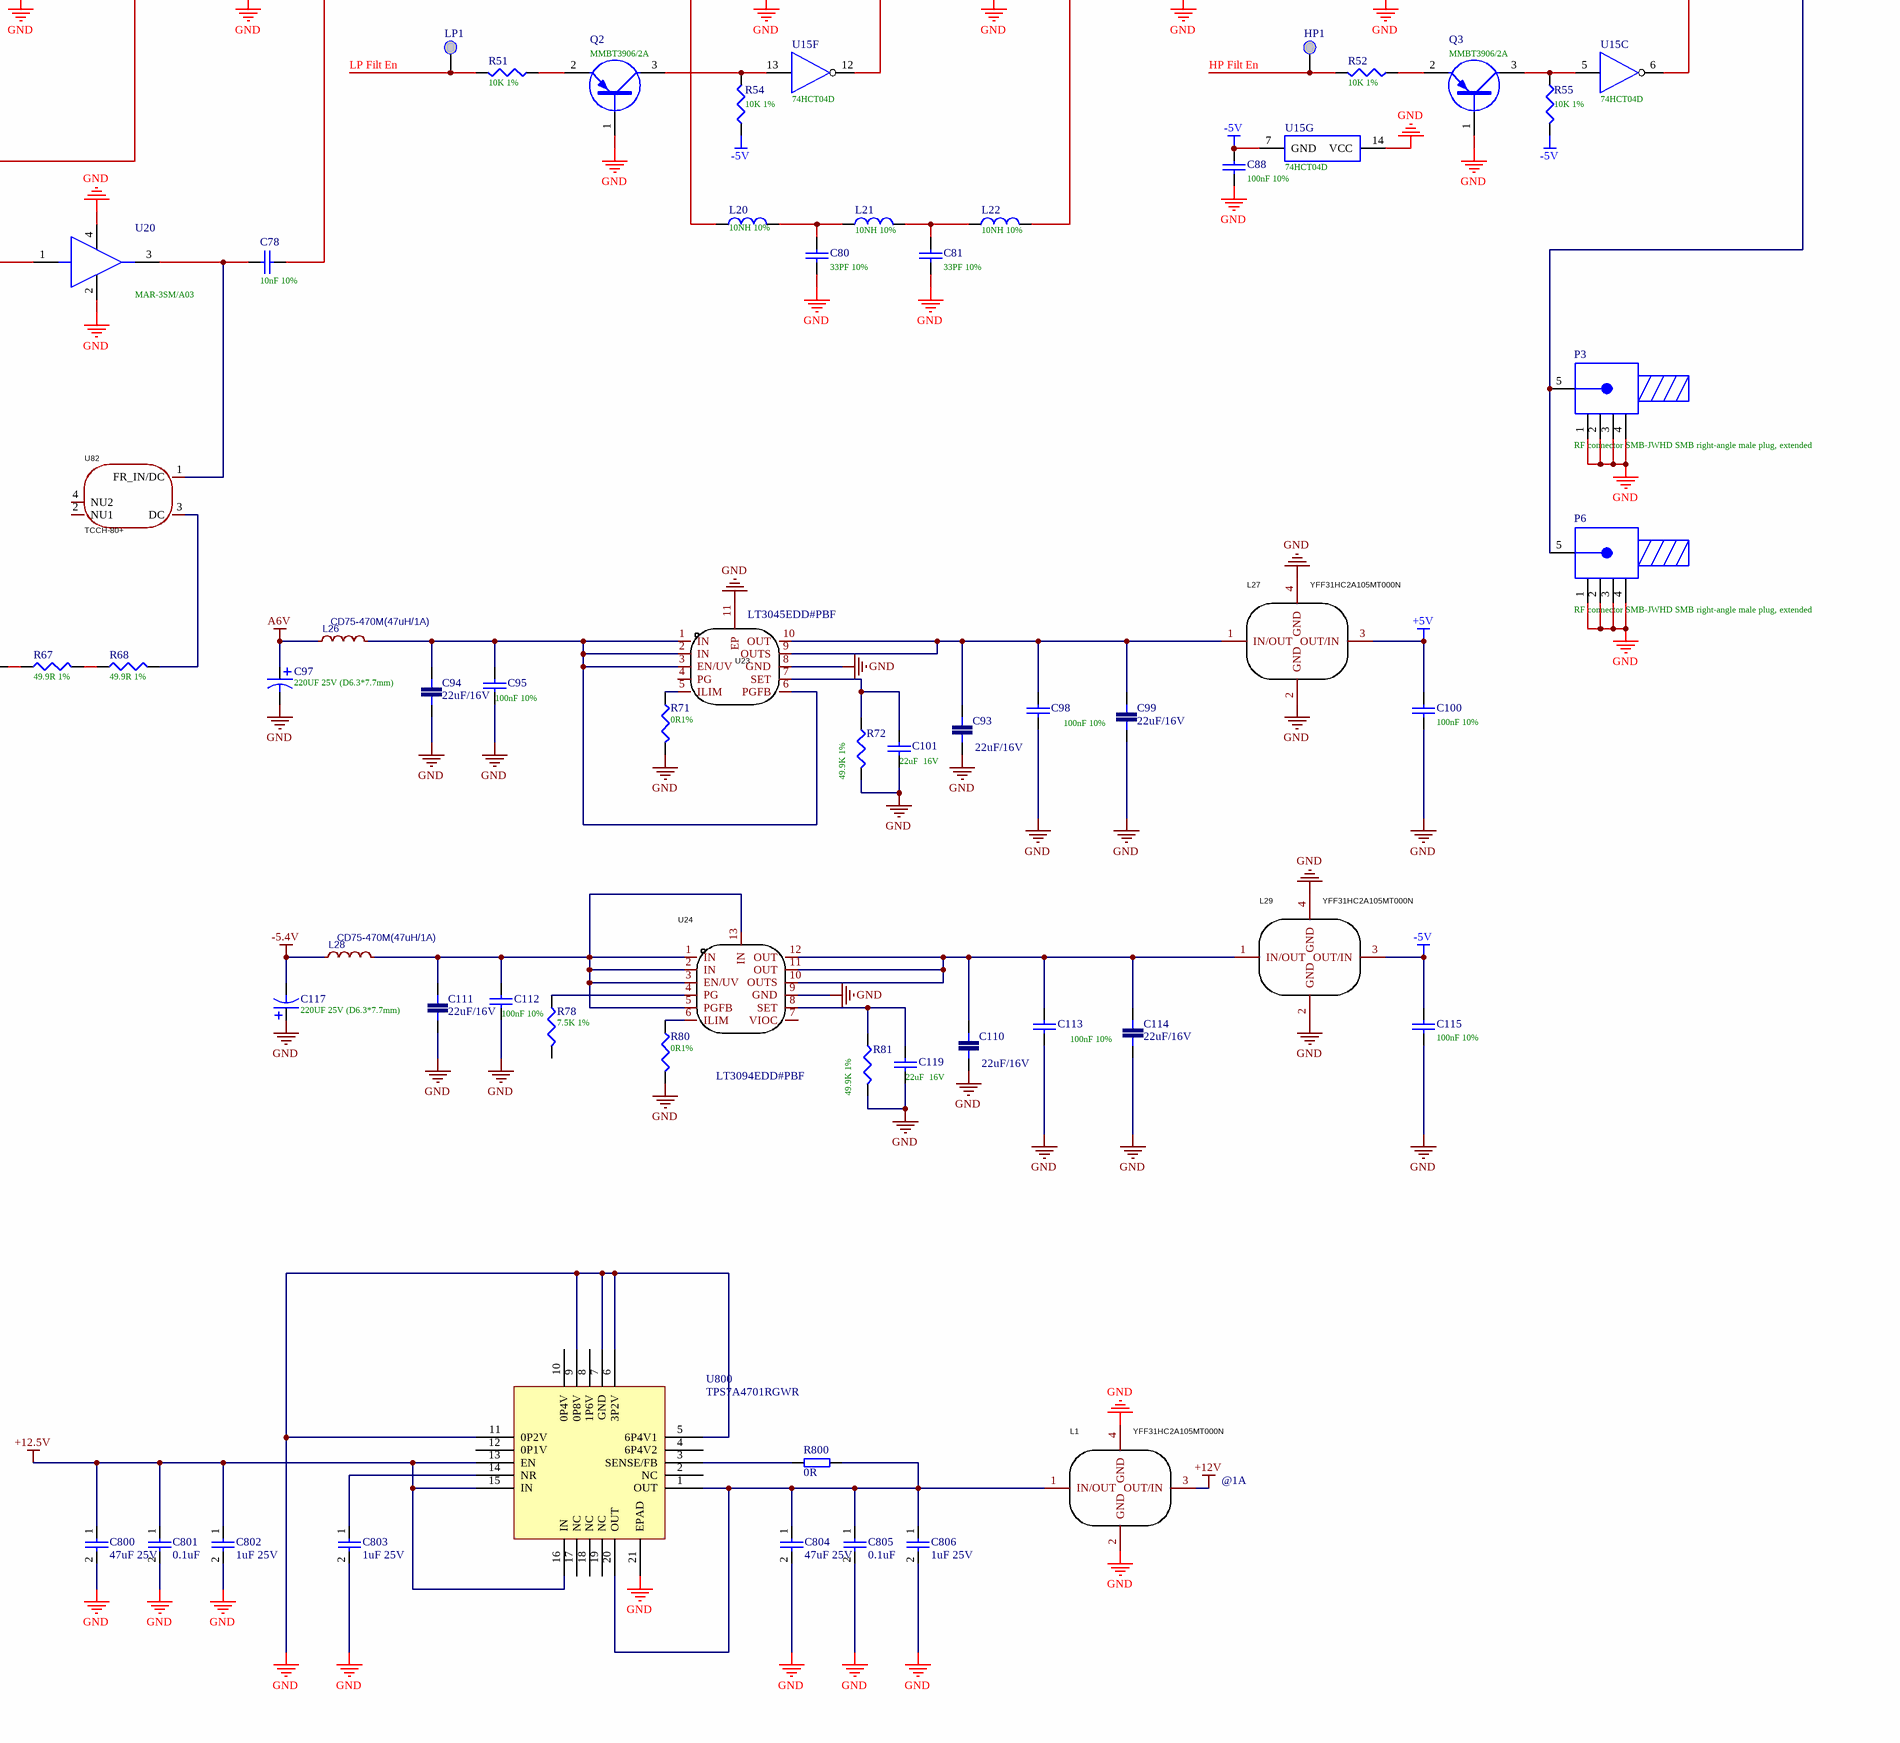
[diagram p0: PCBE109560-11.SchDoc, bottom right]
# Altium schematic sheet PCBE109560-11.SchDoc (part 2 of 2)

## Parts
1  (no value)  [DIP-1]
+1  (no value)  [DIP-1]
+2  (no value)  [DIP-1]
C4  20PF 10%  [0805C]
C5  330PF 10%  [1812C]
C6  22PF 10%  [1812C-2]
C7  22uF/16V  [0805]
C8  22uF/16V  [0805]
C9  100nF 10%  [0603]
C10  220UF 25V (D6.3*7.7mm)  [CAP-SMD_BD6.3-L6.6-W6.6-FD]
C11  100nF 10%  [0603]
C12  22uF/16V  [0805]
C13  100nF 10%  [0805R]
C14  22uF  16V  [0805]
C15  100nF 10%  [0805R]
C16  47PF 10%  [1812C-2]
C17  100PF 10%  [1812C-2]
C18  20PF 10%  [0805R]
C20  100nF 10%  [0805R]
C21  100nF 10%  [0805R]
C31  100nF 10%  [0805R]
C32  100nF 10%  [0805R]
C34  100nF 10%  [0805R]
C35  100nF 10%  [0805R]
C36  100nF 10%  [0805R]
C37  100nF 10%  [0805R]
C39  100nF 10%  [0805R]
C40  100nF 10%  [0805R]
C41  100nF 10%  [0805R]
C42  100nF 10%  [0805R]
C43  100nF 10%  [0805R]
C44  100nF 10%  [0805R]
C45  100nF 10%  [0805R]
C46  100nF 10%  [0805R]
C47  100nF 10%  [0805R]
C48  100nF 10%  [0805R]
C49  22uF 25V  [CAP-SMD_L6.0-W3.2-R-RD]
C50  100nF 10%  [0805R]
C51  100nF 10%  [0805R]
C52  100nF 10%  [0805R]
C53  3.3NF 10%  [0805R]
C54  100nF 10%  [0805R]
C55  330PF 10%  [0805R]
C56  330PF 10%  [0805R]
C57  100nF 10%  [0805R]
C58  33PF 10%  [0805R]
C59  33PF 10%  [0805R]
C60  100nF 10%  [0805R]
C61  100nF 10%  [0805R]
C62  100nF 10%  [0805R]
C63  100nF 10%  [0805R]
C64  100nF 10%  [0805R]
C65  33PF 10%  [0805R]
C66  33PF 10%  [0805R]
C67  100nF 10%  [0805R]
C68  39PF 10%  [0805R]
C69  100nF 10%  [0805R]
C70  25V 1UF Type A  [0805C-2]
C71  25V 1UF Type A  [0805C-2]
C72  100nF 10%  [0805R]
C73  25V 1UF Type A  [0805C-2]
C74  100nF 10%  [0805R]
C75  100nF 10%  [0805R]
C76  10nF 10%  [0805R]
C77  10nF 10%  [0805R]
C78  10nF 10%  [0805R]
C79  100nF 10%  [0603C]
C80  33PF 10%  [0805R]
C81  33PF 10%  [0805R]
C82  100nF 10%  [0805R]
C83  100nF 10%  [0805R]
C84  100nF 10%  [0805R]
C85  100nF 10%  [0805R]
C86  25V 1UF Type A  [0805C-2]
C87  3pF( ±0.1pF)  [0805R]
C88  100nF 10%  [0805R]
C89  100nF 10%  [0805R]
C90  100nF 10%  [0805R]
C93  22uF/16V  [0805]
C94  22uF/16V  [0805]
C95  100nF 10%  [0603]
C96  100nF 10%  [0805R]
C97  220UF 25V (D6.3*7.7mm)  [CAP-SMD_BD6.3-L6.6-W6.6-FD]
C98  100nF 10%  [0603]
C99  22uF/16V  [0805]
C100  100nF 10%  [0805R]
C101  22uF  16V  [0805]
C102  100nF 10%  [0805R]
C103  100nF 10%  [0805R]
C104  100nF 10%  [0805R]
C105  100nF 10%  [0805R]
C106  100nF 10%  [0805R]
C107  100nF 10%  [0805R]
C109  100nF 10%  [0805R]
C110  22uF/16V  [0805]
C111  22uF/16V  [0805]
C112  100nF 10%  [0603]
C113  100nF 10%  [0603]
C114  22uF/16V  [0805]
C115  100nF 10%  [0805R]
C116  100nF 10%  [0805R]
C117  220UF 25V (D6.3*7.7mm)  [CAP-SMD_BD6.3-L6.6-W6.6-FD]
C118  100nF 10%  [0805R]
C119  22uF  16V  [0805]
C122  100nF 10%  [0805R]
C123  100nF 10%  [0805R]
C124  100nF 10%  [0805R]
C125  100nF 10%  [0805R]
C128  100nF 10%  [0805R]
C129  100nF 10%  [0805R]
C130  100nF 10%  [0805R]
C800  47uF 25V  [1206]
C801  0.1uF  [0402]
C802  1uF 25V  [0402]
C803  1uF 25V  [0402]
C804  47uF 25V  [1206]
C805  0.1uF  [0402]
C806  1uF 25V  [0402]
C809  100nF 10%  [0805R]
C888  100nF 10%  [0805R]
Clk1  (no value)  [DIP-1]
D1  BAV99/A7  [SOT-23]
D2  GF1M-E3/67A/GM  [1808D]
D3  GF1M-E3/67A/GM  [1808D]
D4  GF1M-E3/67A/GM  [1808D]
D5  GF1M-E3/67A/GM  [1808D]
D8  BAV99/A7  [SOT-23-2]
D9  BAV99/A7  [SOT-23-2]
D10  BAV99/A7  [SOT-23-2]
D11  BAV99/A7  [SOT-23-2]
D12  BAV99/A7  [SOT-23-2]
Data1  (no value)  [DIP-1]
HP1  (no value)  [DIP-1]
J1  RF connector  [DIP-P]
J2  RF connector  [DIP-P]
L1  YFF31HC2A105MT000N  [FILTER-SMD_4P-L3.2-W1.6-L_YFF31HC]
L2  15UH 5%  [1005R]
L3  BLM21PG221SN1D(220Ω@100MHz)  [0805R]
L4  YFF31HC2A105MT000N  [FILTER-SMD_4P-L3.2-W1.6-L_YFF31HC]
L5  6.8UH 10%  [0805R]
L8  YFF31HC2A105MT000N  [FILTER-SMD_4P-L3.2-W1.6-L_YFF31HC]
L10  10NH 10%  [0805R]
L11  10NH 10%  [0805R]
L12  10NH 10%  [0805R]
L13  YFF31HC2A105MT000N  [FILTER-SMD_4P-L3.2-W1.6-L_YFF31HC]
L15  4.7UH 5%  [1005L]
L16  1UH 5%  [0805R]
L17  BLM21PG221SN1D(220Ω@100MHz)  [0805R]
L18  BLM21PG221SN1D(220Ω@100MHz  [0805R]
L19  NFM15PC104R1A3D  [FILTER-SMD_0402-3P-L1.0-W0.5-T]
L20  10NH 10%  [0805R]
L21  10NH 10%  [0805R]
L22  10NH 10%  [0805R]
L23  YFF31HC2A105MT000N  [FILTER-SMD_4P-L3.2-W1.6-L_YFF31HC]
L24  YFF31HC2A105MT000N  [FILTER-SMD_4P-L3.2-W1.6-L_YFF31HC]
L25  BLM21PG221SN1D(220Ω@100MHz  [0805R]
L26  CD75-470M(47uH/1A)  [IND-SMD_L7.8-W7.0-A]
L27  YFF31HC2A105MT000N  [FILTER-SMD_4P-L3.2-W1.6-L_YFF31HC]
L28  CD75-470M(47uH/1A)  [IND-SMD_L7.8-W7.0-A]
L29  YFF31HC2A105MT000N  [FILTER-SMD_4P-L3.2-W1.6-L_YFF31HC]
L31  BLM21PG221SN1D(220Ω@100MHz  [0805R]
L32  BLM21PG221SN1D(220Ω@100MHz  [0805R]
L808  NFM15PC104R1A3D  [FILTER-SMD_0402-3P-L1.0-W0.5-T]
L809  NFM15PC104R1A3D  [FILTER-SMD_0402-3P-L1.0-W0.5-T]
L810  NFM15PC104R1A3D  [FILTER-SMD_0402-3P-L1.0-W0.5-T]
L811  NFM15PC104R1A3D  [FILTER-SMD_0402-3P-L1.0-W0.5-T]
L812  NFM15PC104R1A3D  [FILTER-SMD_0402-3P-L1.0-W0.5-T]
L813  NFM15PC104R1A3D  [FILTER-SMD_0402-3P-L1.0-W0.5-T]
LP1  (no value)  [DIP-1]
P1  Header 20X2  [N0.8mm/40Pin-Plug]
P2  Header 4X2  [N0.8mm/8Pin-SOCKET]
P3  RF connector SMB-JWHD SMB right-angle male plug, extended  [DIP-P-2]
P4  Header 20X2  [N0.8mm/40Pin-Plug]
P5  Header 20X2  [N0.8mm/40Pin-Plug]
P6  RF connector SMB-JWHD SMB right-angle male plug, extended  [DIP-P-2]
Q1  MJD31C  [SOT-252-2]
Q2  MMBT3906/2A  [SOT-23]
Q3  MMBT3906/2A  [SOT-23]
Q4  MMBT3906/2A  [SOT-23]
R6  2K 5%  [0603R]
R7  NC  [AXIAL-0.51]
R8  3.9K 5% 1/2W  [AXIAL-0.51]
R9  3.9K 5% 1/2W  [AXIAL-0.51]
R10  3.9K 5% 1/2W  [AXIAL-0.51]
R11  3.9K 5% 1/2W  [AXIAL-0.51]
R13  0R1%  [0603]
R14  49.9K 1%  [0603]
R15  4.99K 1%  [0805R]
R16  2K 1%  [0805R]
R17  49.9R 1% 1/4W  [AXIAL-0.4]
R20  100R 1% 1/4W  [AXIAL-0.4]
R23  100R 1% 1/4W  [AXIAL-0.4]
R27  4.87K 1%  [0805R]
R28  4.87K 1%  [0805R]
R29  4.87K 1%  [0805R]
R30  4.87K 1%  [0805R]
R31  4.87K 1%  [0805R]
R32  10K 1%  [0805R]
R33  100K 1%  [0805R]
R34  100K 1%  [0805R]
R35  49.9R 1%  [0805R]
R36  49.9R 1%  [0805R]
R37  49.9R 1%  [0805R]
R38  49.9R 1%  [0805R]
R39  49.9R 1%  [0805R]
R40  49.9R 1% 1/4W  [R-SMD_L3.5-W1.5]
R41  10K 1%  [0805R]
R42  4.87K 1%  [0805R]
R43  4.87K 1%  [0805R]
R44  4.87K 1%  [0805R]
R45  4.87K 1%  [0805R]
R46  169R 1%  [0805R]
R47  169R 1%  [0805R]
R48  169R 1%  [0805R]
R49  49.9R 1%  [0805R]
R50  49.9R 1%  [0805R]
R51  10K 1%  [0805R]
R52  10K 1%  [0805R]
R53  10K 1%  [0805R]
R54  10K 1%  [0805R]
R55  10K 1%  [0805R]
R56  10K 1%  [0805R]
R57  10K 1%  [0805R]
R58  49.9R 1%  [0805R]
R59  4.99K 1%  [0805R]
R60  49.9R 1%  [R-SMD_L3.5-W1.5]
R61  30R 1%  [R-SMD_L3.5-W1.5]
R62  169R 1%  [0805R]
R63  169R 1%  [0805R]
R64  169R 1%  [0805R]
R65  49.9R 1%  [0805R]
R66  49.9R 1%  [0805R]
R67  49.9R 1%  [0805R]
R68  49.9R 1%  [0805R]
R69  120R 1%  [R-SMD_L3.5-W1.5]
R70  169R 1%  [0805R]
R71  0R1%  [0603]
R72  49.9K 1%  [0603]
R73  169R 1%  [0805R]
R74  NC  [0805R]
R75  169R 1%  [0805R]
R77  169R 1%  [0805R]
R78  7.5K 1%  [0603]
R80  0R1%  [0603]
R81  49.9K 1%  [0603]
R82  100K 1%  [0805R]
R83  10K 1%  [0805R]
R84  169R 1%  [0805R]
R800  0R  [0402]
RE1  AGQ210A4HZ  [RELAY-SMD_PANASONIC_AGQ2X0AXX]
RE2  AGQ210A4HZ  [RELAY-SMD_PANASONIC_AGQ2X0AXX]
RE3  AGQ210A4HZ  [RELAY-SMD_PANASONIC_AGQ2X0AXX]
RE4  AGQ210A4HZ  [RELAY-SMD_PANASONIC_AGQ2X0AXX]
RE5  AGQ210A4HZ  [RELAY-SMD_PANASONIC_AGQ2X0AXX]
Strobe1  (no value)  [DIP-1]
U4  LT3045EDD#PBF  [DFN-10_L3.0-W3.0-P0.50-BL-EP]
U6  74HCT123D  [SOIC-16_L9.9-W3.9-P1.27-LS6.0-BL]
U8  MAX504CSD+T  [SO-14]
U9  SW-239  [SO-8]
U11  SW-239  [SO-8]
U12  SW-239  [SO-8]
U13  SW-239  [SO-8]
U14  SW-239  [SO-8]
U15  74HCT04D  [SO-14]  (parts A,B,C,D,E,F,G of 7)
U16  AT-250(MAAV-007941)  [SO-8]
U17  MAR-3SM/A03  [LCC4]
U18  MAR-6SM/A06  [LCC4]
U19  MAR-6SM/A06  [LCC4]
U20  MAR-3SM/A03  [LCC4]
U21  MAX4106ESA+T  [SO-8]
U22  MIC4420CM  [SO-8]
U23  LT3045EDD#PBF  [DFN-10_L3.0-W3.0-P0.50-BL-EP]
U24  LT3094EDD#PBF  [WDFN-12_L3.0-W3.0-P0.45-BL-EP]
U25  AT65-0263  [SO-16]
U80  TCCH-80+  [IND-SMD_4P-L3.8-W3.8]
U81  TCCH-80+  [IND-SMD_4P-L3.8-W3.8]
U82  TCCH-80+  [IND-SMD_4P-L3.8-W3.8]
U83  TCCH-80+  [IND-SMD_4P-L3.8-W3.8]
U100  SW-239  [SO-8]
U800  TPS7A4701RGWR  [QFN-20]

## Nets
+5V: C100.1 C888.1 L25.1 L27.3(OUT/IN) L811.3(OUTPUT) L812.3(OUTPUT) U8.3(~{CLR})
+12.5V: +2.1 C106.1 C800.1 C801.1 C802.1 P5.31 P5.32 P5.33 P5.34 P5.35 P5.36 P5.37 P5.38 P5.39 P5.40 U800.13(EN) U800.15(IN) U800.16(IN)
+12V: C122.1 C123.1 C124.2 C125.2 L1.3(OUT/IN) L8.1(IN/OUT) L13.1(IN/OUT) U22.1(VS) U22.8(VS)
-5.4V: +1.1 C107.1 C117.2 L28.2 P5.1 P5.2 P5.3 P5.4 P5.5 P5.6 P5.7 P5.8 P5.9 P5.10
-5V: C88.2 C115.2 L29.3(OUT/IN) L809.1(INPUT) L810.3(OUTPUT) L813.3(OUTPUT) R54.1 R55.2 R57.1 U15.7(GND)
A6V: 1.1 C10.1 C97.1 C103.2 L3.1 L26.2 P5.17 P5.18 P5.19 P5.20 P5.21 P5.22 P5.23 P5.24
GND: C5.1 C6.2 C7.1 C8.1 C9.2 C10.2 C11.2 C12.1 C13.2 C14.2 C15.1 C18.2 C20.1 C21.1 C31.1 C32.1 C34.1 C35.1 C36.2 C37.2 C39.2 C40.2 C42.2 C43.1 C44.2 C45.2 C46.2 C47.1 C48.1 C49.2 C50.2 C57.2 C60.2 C61.1 C62.1 C63.1 C64.1 C65.2 C66.1 C70.1 C71.1 C72.2 C73.1 C74.1 C75.1 C80.1 C81.1 C83.2 C84.2 C85.1 C86.2 C88.1 C89.2 C90.2 C93.1 C94.1 C95.2 C96.2 C97.2 C98.2 C99.1 C100.2 C101.2 C102.2 C103.1 C104.2 C105.1 C106.2 C107.2 C109.2 C110.1 C111.1 C112.2 C113.2 C114.1 C115.1 C117.1 C118.2 C119.2 C122.2 C123.2 C124.1 C125.1 C128.1 C129.1 C130.2 C800.2 C801.2 C802.2 C803.2 C804.2 C805.2 C806.2 C809.2 C888.2 D1.3 D2.2(K) D11.2 D12.1 J1.1 J1.2 J1.3 J1.4 J2.1 J2.2 J2.3 J2.4 L1.2(GND) L1.4(GND) L2.2 L4.2(GND) L4.4(GND) L8.2(GND) L8.4(GND) L13.2(GND) L13.4(GND) L15.2 L16.1 L19.2(GND) L23.2(GND) L23.4(GND) L24.2(GND) L24.4(GND) L27.2(GND) L27.4(GND) L29.2(GND) L29.4(GND) L808.2(GND) L809.2(GND) L810.2(GND) L811.2(GND) L812.2(GND) L813.2(GND) P1.5 P1.6 P1.11 P1.12 P1.17 P1.18 P1.20 P1.23 P1.24 P1.29 P1.30 P1.35 P1.36 P2.1 P2.3 P2.5 P2.7 P3.1 P3.2 P3.3 P3.4 P4.5 P4.6 P4.11 P4.12 P4.17 P4.18 P4.23 P4.24 P4.29 P4.30 P4.35 P4.36 P5.11 P5.12 P5.13 P5.14 P5.15 P5.16 P5.25 P5.26 P5.27 P5.28 P5.29 P5.30 P6.1 P6.2 P6.3 P6.4 Q1.2(E) Q2.1(B) Q3.1(B) Q4.1(B) R13.2 R14.2 R20.2 R32.2 R53.1 R59.1 R61.1 R71.2 R72.2 R74.1 R80.2 R81.2 R82.1 R83.1 RE1.3 RE3.6 RE4.2 U4.8(GND) U4.11(EP) U6.6(2CEXT) U6.8(GND) U6.10(2B) U6.14(1CEXT) U8.7(DGND) U8.8(AGND) U9.2(GND) U9.7(GND) U9.8(GND) U11.2(GND) U11.7(GND) U11.8(GND) U12.2(GND) U12.7(GND) U12.8(GND) U13.2(GND) U13.7(GND) U13.8(GND) U14.2(GND) U14.7(GND) U14.8(GND) U15.14(VCC) U16.2(GND) U16.3(GND) U16.5(GND) U16.6(GND) U16.7(GND) U17.2(GND) U17.4(GND) U18.2(GND) U18.4(GND) U19.2(GND) U19.4(GND) U20.2(GND) U20.4(GND) U22.4(GND) U22.5(GND) U23.8(GND) U23.11(EP) U24.9(GND) U25.2(GND) U25.3(GND) U25.4(GND) U25.5(GND) U25.6(GND) U25.7(GND) U25.16(GND) U100.2(GND) U100.7(GND) U100.8(GND) U800.5(6P4V1) U800.6(3P2V) U800.7(GND) U800.9(0P8V) U800.11(0P2V) U800.21(EPAD)
VCC: C13.1 C15.2 L4.3(OUT/IN) R15.1 R16.2 U6.2(1B) U6.3(1~{R}D) U6.16(VCC)
AK2: C21.2 P1.33 RE1.1
AK3: C20.2 P1.38 RE1.8
AK4: C37.1 P1.37 RE2.1
AK5: C36.1 P1.40 RE2.8
AK6: C31.2 P1.34 RE3.8
AK7: C32.2 P1.32 RE3.1
AK8: C34.2 C40.1 P1.28 RE4.8 RE5.8
AK9: C35.2 C39.1 P1.26 RE4.1 RE5.1
Attn1: P4.34 R70.2
Attn2: P4.32 R73.2
Attn4: P4.28 R75.2
Attn8: P4.26 R77.2
Attn16: P4.22 R84.2
DAC Clk: Clk1.1 P4.14 U8.4(SCLK)
DAC Data: Data1.1 P4.16 U8.2(DIN)
DAC Strobe: P4.10 Strobe1.1 U8.5(~{CS})
DATA_T: P1.39 R15.2 U6.1(1~{A})
HP Filt En: HP1.1 P4.4 R52.2
HT: L5.1 P2.2 P2.4 P2.6 P2.8
IN2: P4.8 R56.1 U22.2(IN)
LP Filt En: LP1.1 P4.2 R51.2
NetC4_1: C4.1 D1.2 L2.1 Q1.1(B) R6.1
NetC4_2: C4.2 R6.2 U6.13(1Q)
NetC5_2: C5.2 L5.2 R7.2
NetC6_1: C6.1 C16.2 C17.2 Q1.3(C) R11.1
NetC7_2: C7.2 C11.1 C12.2 L4.1(IN/OUT) U4.9(OUTS) U4.10(OUT)
NetC8_2: C8.2 C9.1 L3.2 U4.1(IN) U4.2(IN) U4.3(EN/UV) U4.6(PGFB)
NetC14_1: C14.1 R14.1 U4.7(SET)
NetC16_1: C16.1 D5.1(A) D8.2 D9.2 RE2.6
NetC17_1: C17.1 RE2.7
NetC18_1: C18.1 R16.1 U6.15(1REXT/CEXT)
NetC41_1: C41.1 U14.1(RFCOM)
NetC41_2: C41.2 P3.5 P6.5 R32.1
NetC42_1: C42.1 R27.1 U9.5(B)
NetC43_2: C43.2 R28.2 U100.4(A)
NetC44_1: C44.1 R29.1 U11.4(A)
NetC45_1: C45.1 R30.1 U12.5(B)
NetC46_1: C46.1 R31.1 U13.5(B) U14.4(A)
NetC47_2: C47.2 R35.1 U16.4(A)
NetC48_2: C48.2 L8.3(OUT/IN) R36.1
NetC49_1: C49.1 C50.1 U8.1(BIPOFF) U8.9(REFIN) U8.10(REFOUT)
NetC51_1: C51.1 U17.1(RF_IN)
NetC51_2: C51.2 U16.8(RF2)
NetC52_1: C52.1 L10.2
NetC52_2: C52.2 U17.3(RF_OUT) U81.1(FR_IN/DC)
NetC53_1: C53.1 C54.1 L15.1
NetC53_2: C53.2 U12.1(RFCOM)
NetC54_2: C54.2 U13.1(RFCOM)
NetC55_1: C55.1 U13.3(RF1)
NetC55_2: C55.2 C56.1 L16.2
NetC56_2: C56.2 U14.6(RF2)
NetC57_1: C57.1 R41.1 U13.4(A) U14.5(B)
NetC58_1: C58.1 C65.1
NetC58_2: C58.2 L10.1 L11.1
NetC59_1: C59.1 L11.2 L12.1
NetC59_2: C59.2 C66.2
NetC60_1: C60.1 R42.1 U9.4(A)
NetC61_2: C61.2 R43.2 U100.5(B)
NetC62_2: C62.2 R44.1 U11.5(B)
NetC63_2: C63.2 R45.1 U12.4(A)
NetC64_2: C64.2 L13.3(OUT/IN) R46.2
NetC67_1: C67.1 U18.1(RF_IN)
NetC67_2: C67.2 U25.1(RF)
NetC68_1: C68.1 C69.2 R49.2 R50.2
NetC68_2: C68.2 R49.1 R50.1 U18.3(RF_OUT) U80.1(FR_IN/DC)
NetC69_1: C69.1 R53.2 U16.1(RF1)
NetC70_2: C70.2 C74.2 L18.1 L19.1(INPUT)
NetC71_2: C71.2 C75.2 L19.3(OUTPUT) U21.4(VEE)
NetC72_1: C72.1 C73.2 L17.2 L18.2
NetC76_1: C76.1 U9.3(RF1)
NetC76_2: C76.2 U19.1(RF_IN)
NetC77_1: C77.1 U19.3(RF_OUT) U83.1(FR_IN/DC)
NetC77_2: C77.2 U20.1(RF_IN)
NetC78_1: C78.1 U20.3(RF_OUT) U82.1(FR_IN/DC)
NetC78_2: C78.2 U100.6(RF2)
NetC79_1: C79.1 D10.3 R40.2
NetC79_2: C79.2 R58.2 R59.2
NetC80_2: C80.2 L20.2 L21.2
NetC81_2: C81.2 L21.1 L22.1
NetC82_1: C82.1 R60.2
NetC82_2: C82.2 C116.1 R74.2 R82.2
NetC83_1: C83.1 C86.1 L808.1(INPUT) U21.7(VCC)
NetC84_1: C84.1 L23.3(OUT/IN) R62.2
NetC85_2: C85.2 L24.3(OUT/IN) R65.1
NetC87_1: C87.1 R60.1 R69.1 U21.6(OUT)
NetC87_2: C87.2 R61.2 R69.2 U21.2(IN-)
NetC89_1: C89.1 L813.1(INPUT) U8.11(VSS)
NetC90_1: C90.1 L32.2 L811.1(INPUT)
NetC93_2: C93.2 C98.1 C99.2 L27.1(IN/OUT) U23.9(OUTS) U23.10(OUT)
NetC94_2: C94.2 C95.1 L26.1 U23.1(IN) U23.2(IN) U23.3(EN/UV) U23.6(PGFB)
NetC96_1: C96.1 R70.1 U25.15(C1)
NetC101_1: C101.1 R72.1 U23.7(SET)
NetC102_1: C102.1 R73.1 U25.14(C2)
NetC104_1: C104.1 L812.1(INPUT) U8.13(VDD)
NetC105_2: C105.2 L31.1 L810.1(INPUT)
NetC109_1: C109.1 R75.1 U25.13(C4)
NetC110_2: C110.2 C113.1 C114.2 L29.1(IN/OUT) U24.10(OUTS) U24.11(OUT) U24.12(OUT)
NetC111_2: C111.2 C112.1 L28.1 U24.1(IN) U24.2(IN) U24.3(EN/UV) U24.5(PGFB) U24.13(IN)
NetC116_2: C116.2 R83.2 U25.8(RF)
NetC118_1: C118.1 R77.1 U25.12(C8)
NetC119_1: C119.1 R81.1 U24.8(SET)
NetC128_2: C128.2 L31.2 U25.11(VEE)
NetC129_2: C129.2 L32.1 U25.10(VCC)
NetC130_1: C130.1 R84.1 U25.9(C16)
NetC803_1: C803.1 U800.14(NR)
NetC804_1: C804.1 C805.1 C806.1 L1.1(IN/OUT) R800.1 U800.1(OUT) U800.20(OUT)
NetC809_1: C809.1 L25.2 L808.3(OUTPUT)
NetD2_1: D2.1(A) D3.2(K)
NetD3_1: D3.1(A) D4.2(K)
NetD4_1: D4.1(A) D5.2(K)
NetD8_1: D8.1 D9.1 J1.5 R17.1 R20.1 R23.1 RE4.4
NetD10_1: D10.1 D12.2
NetD10_2: D10.2 D11.1
NetJ2_5: J2.5 RE5.4
NetL12_2: L12.2 U9.1(RFCOM)
NetL17_1: L17.1 L809.3(OUTPUT)
NetL20_1: L20.1 U11.6(RF2)
NetL22_2: L22.2 U12.3(RF1)
NetL23_1: L23.1(IN/OUT) L24.1(IN/OUT) U22.6(OUT) U22.7(OUT)
NetQ2_2: Q2.2(E) R51.1
NetQ2_3: Q2.3(C) R54.2 U15.13(6A)
NetQ3_2: Q3.2(E) R52.1
NetQ3_3: Q3.3(C) R55.1 U15.5(3A)
NetQ4_2: Q4.2(E) R56.2
NetQ4_3: Q4.3(C) R57.2 U15.1(1A)
NetR7_1: R7.1 R8.1
NetR8_2: R8.2 R9.2
NetR9_1: R9.1 R10.1
NetR10_2: R10.2 R11.2
NetR13_1: R13.1 U4.5(ILIM)
NetR17_2: R17.2 RE1.2
NetR23_2: R23.2 RE3.7
NetR27_2: R27.2 R28.1 U15.4(2Y)
NetR29_2: R29.2 R30.2 U15.10(5Y)
NetR31_2: R31.2 U15.8(4Y)
NetR33_1: R33.1 R34.1 U8.14(RFB)
NetR33_2: R33.2 R34.2 R35.2 U8.12(VOUT)
NetR36_2: R36.2 R37.1
NetR37_2: R37.2 R38.2
NetR38_1: R38.1 R39.1
NetR39_2: R39.2 U81.3(DC)
NetR40_1: R40.1 RE5.3
NetR41_2: R41.2 U15.6(3Y) U15.9(4A)
NetR42_2: R42.2 R43.1 U15.2(1Y) U15.3(2A)
NetR44_2: R44.2 R45.2 U15.11(5A) U15.12(6Y)
NetR46_1: R46.1 R47.2
NetR47_1: R47.1 R48.1
NetR48_2: R48.2 U80.3(DC)
NetR58_1: R58.1 U21.3(IN+)
NetR62_1: R62.1 R63.1
NetR63_2: R63.2 R64.2
NetR64_1: R64.1 U83.3(DC)
NetR65_2: R65.2 R66.2
NetR66_1: R66.1 R67.1
NetR67_2: R67.2 R68.1
NetR68_2: R68.2 U82.3(DC)
NetR71_1: R71.1 U23.5(ILIM)
NetR78_1: R78.1 U24.4(PG)
NetR80_1: R80.1 U24.6(ILIM)
NetR800_2: R800.2 U800.3(SENSE/FB)
NetRE4_3: RE4.3 RE5.2
NetU9_6: U9.6(RF2) U100.3(RF1)
NetU11_1: U11.1(RFCOM) U100.1(RFCOM)
NetU11_3: U11.3(RF1) U12.6(RF2)
NetU13_6: U13.6(RF2) U14.3(RF1)

Not connected (* = marked no-connect by the designer): D1 1*; D8 3; D9 3; D11 3; D12 3; P1 1 2 3 4 7 8 9 10 13 14 15 16 19 21 22 25 27 31; P4 1 3 7 9 13 15 19 20 21 25 27 31 33 37 38 39 40; R78 2; RE1 4 5 6 7; RE2 2 3 4 5; RE3 2 3 4 5; RE4 5 6 7; RE5 5 6 7; U4 4(PG); U6 4(1~{Q}) 5(2Q) 7(2REXT/CEXT) 9(2~{A}) 11(2~{R}D) 12(2~{Q}); U8 6(DOUT); U22 3(NC); U23 4(PG); U24 7(VIOC); U80 2(NU1) 4(NU2); U81 2(NU1) 4(NU2); U82 2(NU1) 4(NU2); U83 2(NU1) 4(NU2); U800 2(NC) 4(6P4V2) 8(1P6V) 10(0P4V) 12(0P1V) 17(NC) 18(NC) 19(NC)

## Notes on the sheet
- (near P1) Transmit interface
- 500V high-voltage interface
- Receive interface
- @1A

## Library data of the parts
1 +1 +2 Clk1 Data1 HP1 LP1 Strobe1 = TP
C4-C6 C9 C11 C13-C18 C20 C21 C31 C32 C34-C37 C39-C48 C50-C69 C72-C85 C87-C90 C95 C96 C98 C100-C107 C109 C112 C113 C115 C116 C118 C119 C122-C125 C128-C130 C800-C806 C809 C888 = CAP: Capacitor
C7 C8 C12 C93 C94 C99 C110 C111 C114 = C1206
C10 C97 C117 = CAPACITOR_1: Capacitor
C49 = TAJC226K025RNJ: Manufacturer: Kyocera AVX; Add into BOM: yes; Tolerance: ±10%; Equivalent Series Resistance(ESR): 1.4Ω@100kHz; Symbol: TAJC226K025RNJ; Device: TAJC226K025RNJ; LCSC Part Name: 22uF ±10% 25V; Supplier Part: C7214; Manufacturer Part: TAJC226K025RNJ; Supplier Footprint: CASE-C-6032; JLCPCB Part Class: Extended Part; Datasheet: https://atta.szlcsc.com/upload/public/pdf/source/20160107/1457707750344.pdf; Supplier: LCSC; Convert to PCB: yes; Value: 22uF; Rated Voltage: 25V; Operating Temperature: -55℃~+125℃
C70 C71 C86 = CAPACITOR POL: Capacitor
D1 D8-D12 = BAV99
D2-D5 = DIODE
J1 J2 = SMA-KWE: BOM_Supplier: *; BOM_Supplier Part: *; BOM_Manufacturer: *; BOM_Manufacturer Part: *; BOM_JLCPCB Part Class: *; spicePre: *; spiceSymbolName: *; Contributor: *
L1 L4 L8 L13 L23 L24 L27 L29 = YFF31HC2A105MT000N: Manufacturer: TDK; Add into BOM: yes; Nominal Capacitance: 1uF; CapacitanceTolerance: ±20%; DC Rated Voltage: 100V; Rated Current: 6A; DC Resistance: 5mΩ; Name: YFF31HC2A105MT000N; Symbol: YFF31HC2A105MT000N; Device: YFF31HC2A105MT000N; LCSC Part Name: 1uF(105) ±20% 100V; Supplier Part: C113216; Manufacturer Part: YFF31HC2A105MT000N; Supplier Footprint: SMD-4P,1.6x3.2mm; JLCPCB Part Class: Extended Part; Datasheet: https://atta.szlcsc.com/upload/public/pdf/source/20180326/C113216_F6F81E50B9805DA3D7C436129903DEBD.pdf; Supplier: LCSC; Convert to PCB: yes; Operating Temperature: -55℃~+125℃
L2 L3 L5 L10-L12 L15-L18 L20-L22 L25 L31 L32 = INDUCTOR
L19 L808-L813 = NFM15PC104R1A3D: Manufacturer: muRata(村田); Add into BOM: yes; Nominal Capacitance: 100nF; CapacitanceTolerance: ±20%; DC Rated Voltage: 10V; Rated Current: 2A; DC Resistance: 30mΩ; Symbol: NFM15PC104R1A3D; Device: NFM15PC104R1A3D; LCSC Part Name: 0.1uF ±20% 10V; Supplier Part: C2650905; Manufacturer Part: NFM15PC104R1A3D; Supplier Footprint: 0402; JLCPCB Part Class: Extended Part; Datasheet: https://atta.szlcsc.com/upload/public/pdf/source/20210611/05FD8D968916F804F398094FB2B4AAFE.pdf; Supplier: LCSC; Convert to PCB: yes; Operating Temperature: -55℃~+105℃; Comment_1: NFM15PC104R1A3D
L26 L28 = 4.7uH/5a: BOM_Manufacturer: COILMX; BOM_Manufacturer Part: MS0630-4R7M; nameAlias: Inductance; Contributor: LCSC; BOM_Supplier: LCSC; BOM_Supplier Part: C380177; spicePre: L; spiceSymbolName: MS0630-4R7M
P1 P4 P5 = Header 20X2: Header, 20-Pin, Dual row; LatestRevisionDate: 17-Jul-2002; LatestRevisionNote: Re-released for DXP Platform.; Publisher: Altium Limited
P2 = Header 4X2: Header, 4-Pin, Dual row; LatestRevisionDate: 17-Jul-2002; LatestRevisionNote: Re-released for DXP Platform.; Publisher: Altium Limited
P3 P6 = JA1
Q1 = NPN: NPN Transistor
Q2-Q4 = PNP: PNP Transistor
R6-R11 R13-R17 R20 R23 R27-R75 R77 R78 R80-R84 = RES1
R800 = RES
RE1-RE5 = AGQ210A4HZ: Manufacturer: PANASONIC(松下); Add into BOM: yes; Coil Voltage: 4.5V; Contact Form: Two changeover sets: 2C (DPDT changeover); Maximum Switching Voltage: 125V@AC; 110V@DC; Coil Type: Single coil; Maximum Switching Current: 2A; Operate Time: 4ms; Symbol: AGQ210A4HZ; Device: AGQ210A4HZ; LCSC Part Name: AGQ210A4HZ; Supplier Part: C2153577; Manufacturer Part: AGQ210A4HZ; Supplier Footprint: SMD,7.2x10.6mm; JLCPCB Part Class: Extended Part; Datasheet: https://atta.szlcsc.com/upload/public/pdf/source/20210727/C2858037_82AE1FE69E1888D41D6E9B5D42950540.pdf; Supplier: LCSC; Convert to PCB: yes; Pin Number: -; Contact Rating: -; Contact Material: AgPd + gold plating; Coil Rated Power: -; Coil Resistance: -; Release Time: 4ms; Contact Resistance: -; Operating Temperature: -40℃~+85℃; Comment_1: AGQ210A4HZ
U4 U23 = LT3045EDD#PBF: Symbol: LT3045EDD#PBF_C666574; Add into BOM: yes; Maximum Input Voltage: 20V; Output Voltage: 0V~15V; MAX Output Current: 500mA; Dropout Voltage: 450mV@(500mA); standby current: 20uA; Number of Outputs: 1; Device: LT3045EDD#PBF; LCSC Part Name: LT3045EDD#PBF; Supplier Part: C666574; Manufacturer Part: LT3045EDD#PBF; Supplier Footprint: DFN-10-EP(3x3); JLCPCB Part Class: Extended Part; Datasheet: https://atta.szlcsc.com/upload/public/pdf/source/20200416/C514420_E440C492D6C74EAE6AB301243586F696.pdf; Supplier: LCSC; Convert to PCB: yes
U15 = 74HC04
U16 = AT-250
U17 U20 = MAR-3SM
U18 U19 = MAR-6SM
U21 = MAX4107ESA: Manufacturer: *; Manufacturer Part: *; Supplier Part: *; Supplier: *; link: *; spicePre: *; spiceSymbolName: *; Package Display: *; Contributor: *
U24 = LT3094EDD#PBF: Add into BOM: yes; Symbol: LT3094EDD#PBF; Device: LT3094EDD#PBF; LCSC Part Name: LT3094EDD#PBF; Supplier Part: C670492; Manufacturer Part: LT3094EDD#PBF; Supplier Footprint: WDFN-12-EP(3x3); JLCPCB Part Class: Extended Part; Datasheet: https://atta.szlcsc.com/upload/public/pdf/source/20200318/C498217_A5485280C797CF3891C55BEBE66C21D4.pdf; Supplier: LCSC; Convert to PCB: yes; Output Type: -
U80-U83 = TCCH-80+: Manufacturer: Mini-Circuits; Add into BOM: yes; Value: 4uH; Rated Current: 200mA; DC Resistance (DCR): 100mΩ; Symbol: TCCH-80+; Device: TCCH-80+; LCSC Part Name: 4uH; Supplier Part: C3223029; Manufacturer Part: TCCH-80+; Supplier Footprint: SMD-4P,3.8x3.8mm; JLCPCB Part Class: Extended Part; Datasheet: https://atta.szlcsc.com/upload/public/pdf/source/20240402/75EC49D4FFFA61CBEC009CC2CCA83C83.pdf; Supplier: LCSC; Convert to PCB: yes; Tolerance: -; Saturation Current (Isat): -; Type: -; Ratings: -
U800 = TPS7A4701RGWR(QFN20): Name: *; Symbol: *; Device: *; LCSC Part Name: *; Supplier Part: *; Manufacturer: *; Manufacturer Part: *; Supplier Footprint: *; JLCPCB Part Class: *; Datasheet: *; Supplier: *; Add into BOM: *; Convert to PCB: *; Output Type: *; Output Polarity: *; Number of Outputs: *